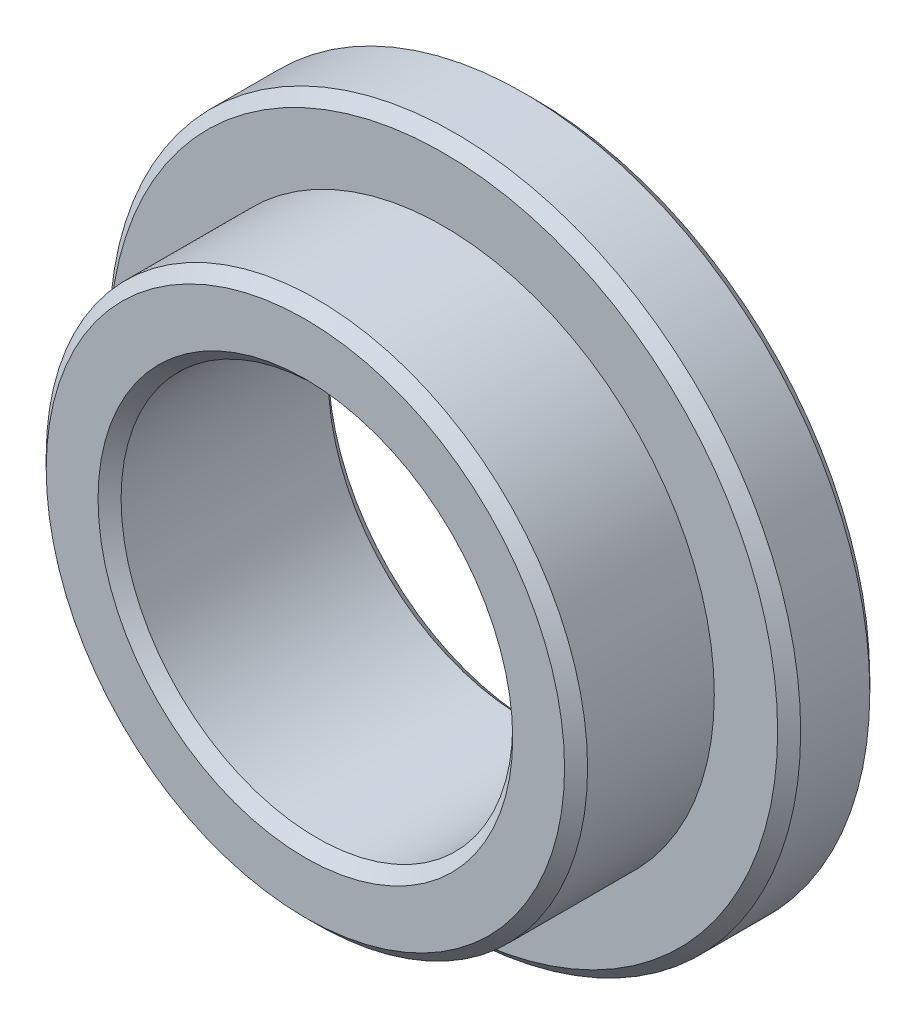
SolidWorks part; units mm, degrees
ref_plane "Front Plane" through (0, 0, 0) normal (0, 0, 1) x (1, 0, 0)
ref_plane "Top Plane" through (0, 0, 0) normal (0, 1, 0) x (1, 0, 0)
ref_plane "Right Plane" through (0, 0, 0) normal (1, 0, 0) x (0, 0, -1)
other "Configuration Table"
sketch "Sketch1" plane through (0, 0, 0) normal (0, 0, 1) x (1, 0, 0)
  circle A0 centre (0, 0) radius 15
  dimension "D1" = 30
extrude "Boss-Extrude1" add sketch "Sketch1" along normal blind 4
sketch "Sketch2" plane through (0, 0, 4) normal (0, 0, 1) x (1, 0, 0)
  circle A0 centre (0, 0) radius 11.75
  dimension "D1" = 23.5
extrude "Boss-Extrude2" add sketch "Sketch2" along normal blind 6
sketch "Sketch3" plane through (0, 0, 0) normal (0, 0, -1) x (-1, 0, 0)
  circle A0 centre (0, 0) radius 8.5
  dimension "D1" = 17
extrude "Cut-Extrude1" cut sketch "Sketch3" against normal blind 20
chamfer "Chamfer1" distance 0.5 angle 45 2 edges at (-8.5, 0, 0) (8.5, 0, 10)
chamfer "Chamfer2" distance 0.5 angle 45 3 edges at (15, 0, 0) (15, 0, 4) (11.75, 0, 10)
